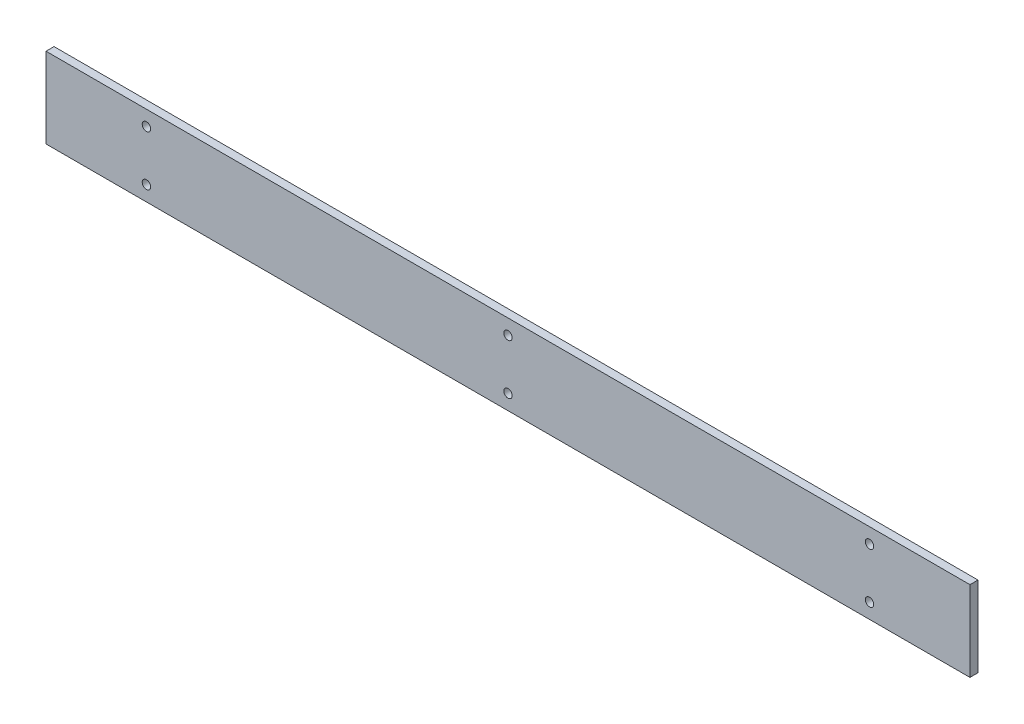
SolidWorks part; units mm, degrees
material "不锈钢 (铁素体)"
ref_plane "前视基准面" through (0, 0, 0) normal (0, 0, 1) x (1, 0, 0)
ref_plane "上视基准面" through (0, 0, 0) normal (0, 1, 0) x (1, 0, 0)
ref_plane "右视基准面" through (0, 0, 0) normal (1, 0, 0) x (0, 0, -1)
sketch "草图1" plane through (0, 0, 0) normal (0, 0, 1) x (1, 0, 0)
  line L1 (-230, 20) -> (230, 20)
  line L2 (-230, 20) -> (-230, -20)
  line L3 (-230, -20) -> (230, -20)
  line L4 (230, 20) -> (230, -20)
  line L5 (-230, 20) -> (230, -20) construction
  line L6 (-230, -20) -> (230, 20) construction
  point P0 (0, 0)
  dimension "D1" = 460
  dimension "D2" = 40
extrude "凸台-拉伸1" add sketch "草图1" along normal mid plane 4
hole_wizard "M5 螺纹孔1" positions "草图3" profile "草图2" tap size "M5" standard "GB"
sketch "草图3" plane through (0, 0, 2) normal (0, 0, 1) x (1, 0, 0)
  point P0 (-180, 12.5)
  point P2 (-180, -12.5)
  point P4 (0, 12.5)
  point P6 (0, -12.5)
  point P8 (180, 12.5)
  point P10 (180, -12.5)
  dimension "D1" = 180
  dimension "D2" = 180
  dimension "D3" = 25
  dimension "D4" = 12.5
sketch "草图2" plane through (-180, 12.5, 2) normal (1, 0, 0) x (0, -1, 0)
  line L0 (0, 0) -> (0, 15.2618)
  line L1 (0, 15.2618) -> (2.1, 14)
  line L2 (2.1, 14) -> (2.1, 0)
  line L5 (2.1, 0) -> (0, 0)
  line L10 (0, 15.2618) -> (-2.1, 14) construction
  line L11 (0, -6.35) -> (0, 107.95) construction
  dimension "螺纹孔钻头直径" = 4.2
  dimension "螺纹孔钻头深度" = 14
  dimension "导头角度" = 118
cosmetic thread "孔螺蚊线1"
cosmetic thread "孔螺蚊线2"
cosmetic thread "孔螺蚊线3"
cosmetic thread "孔螺蚊线4"
cosmetic thread "孔螺蚊线5"
cosmetic thread "孔螺蚊线6"
